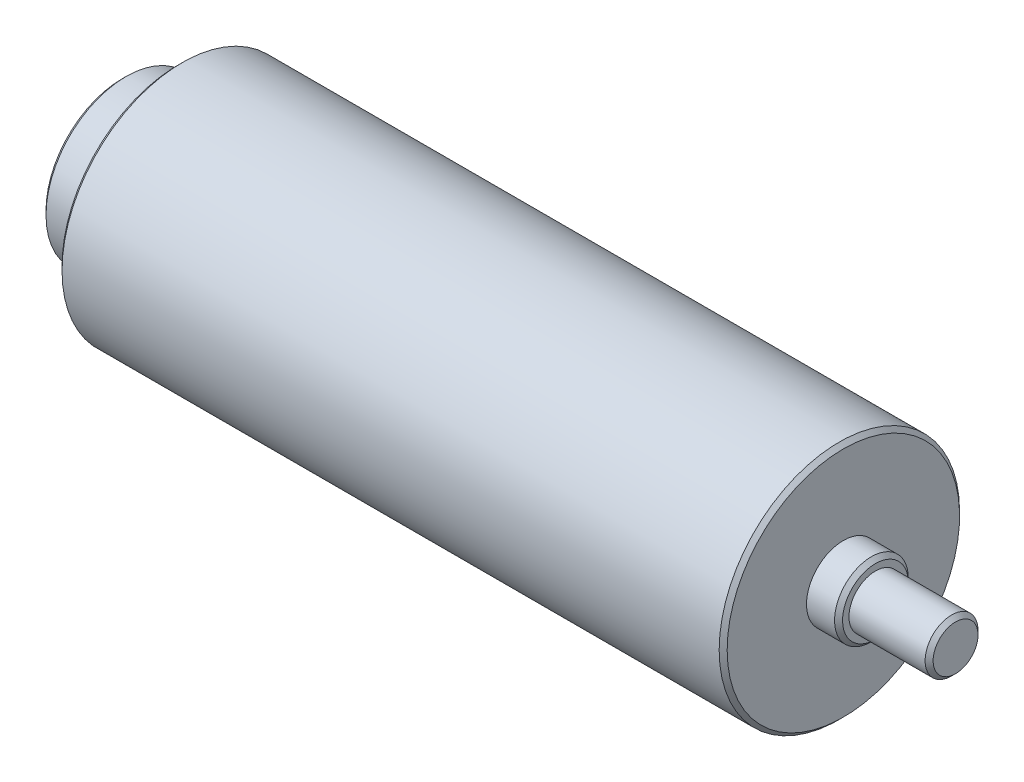
from build123d import *

# Parameters (mm, degrees)
CHAMFER1_SIZE = 0.5


with BuildPart() as part:
    # Sketch1 → Revolve1 (revolve)
    with BuildSketch(Plane.XY):
        Polygon((695.508784709, 30.649610335), (685.508784709, 30.649610335), (685.508784709, 31.949610335), (681.508784709, 31.949610335), (681.508784709, 42.349610335), (598.508784709, 42.349610335), (598.508784709, 37.349610335), (591.508784709, 37.349610335), (591.508784709, 27.349610335), (695.508784709, 27.349610335), align=None)
    revolve(axis=Axis((695.508784709, 27.349610335, 0), (-1, 0, 0)))

    # Chamfer1
    chamfer1_edges = [part.edges().sort_by_distance(p)[0] for p in [
        (695.508784709, 24.049610335, 0),
        (685.508784709, 22.749610335, 0),
        (681.508784709, 12.349610335, 0),
        (598.508784709, 12.349610335, 0),
        (591.508784709, 17.349610335, 0),
    ]]
    chamfer(chamfer1_edges, length=CHAMFER1_SIZE)


solid = part.part
